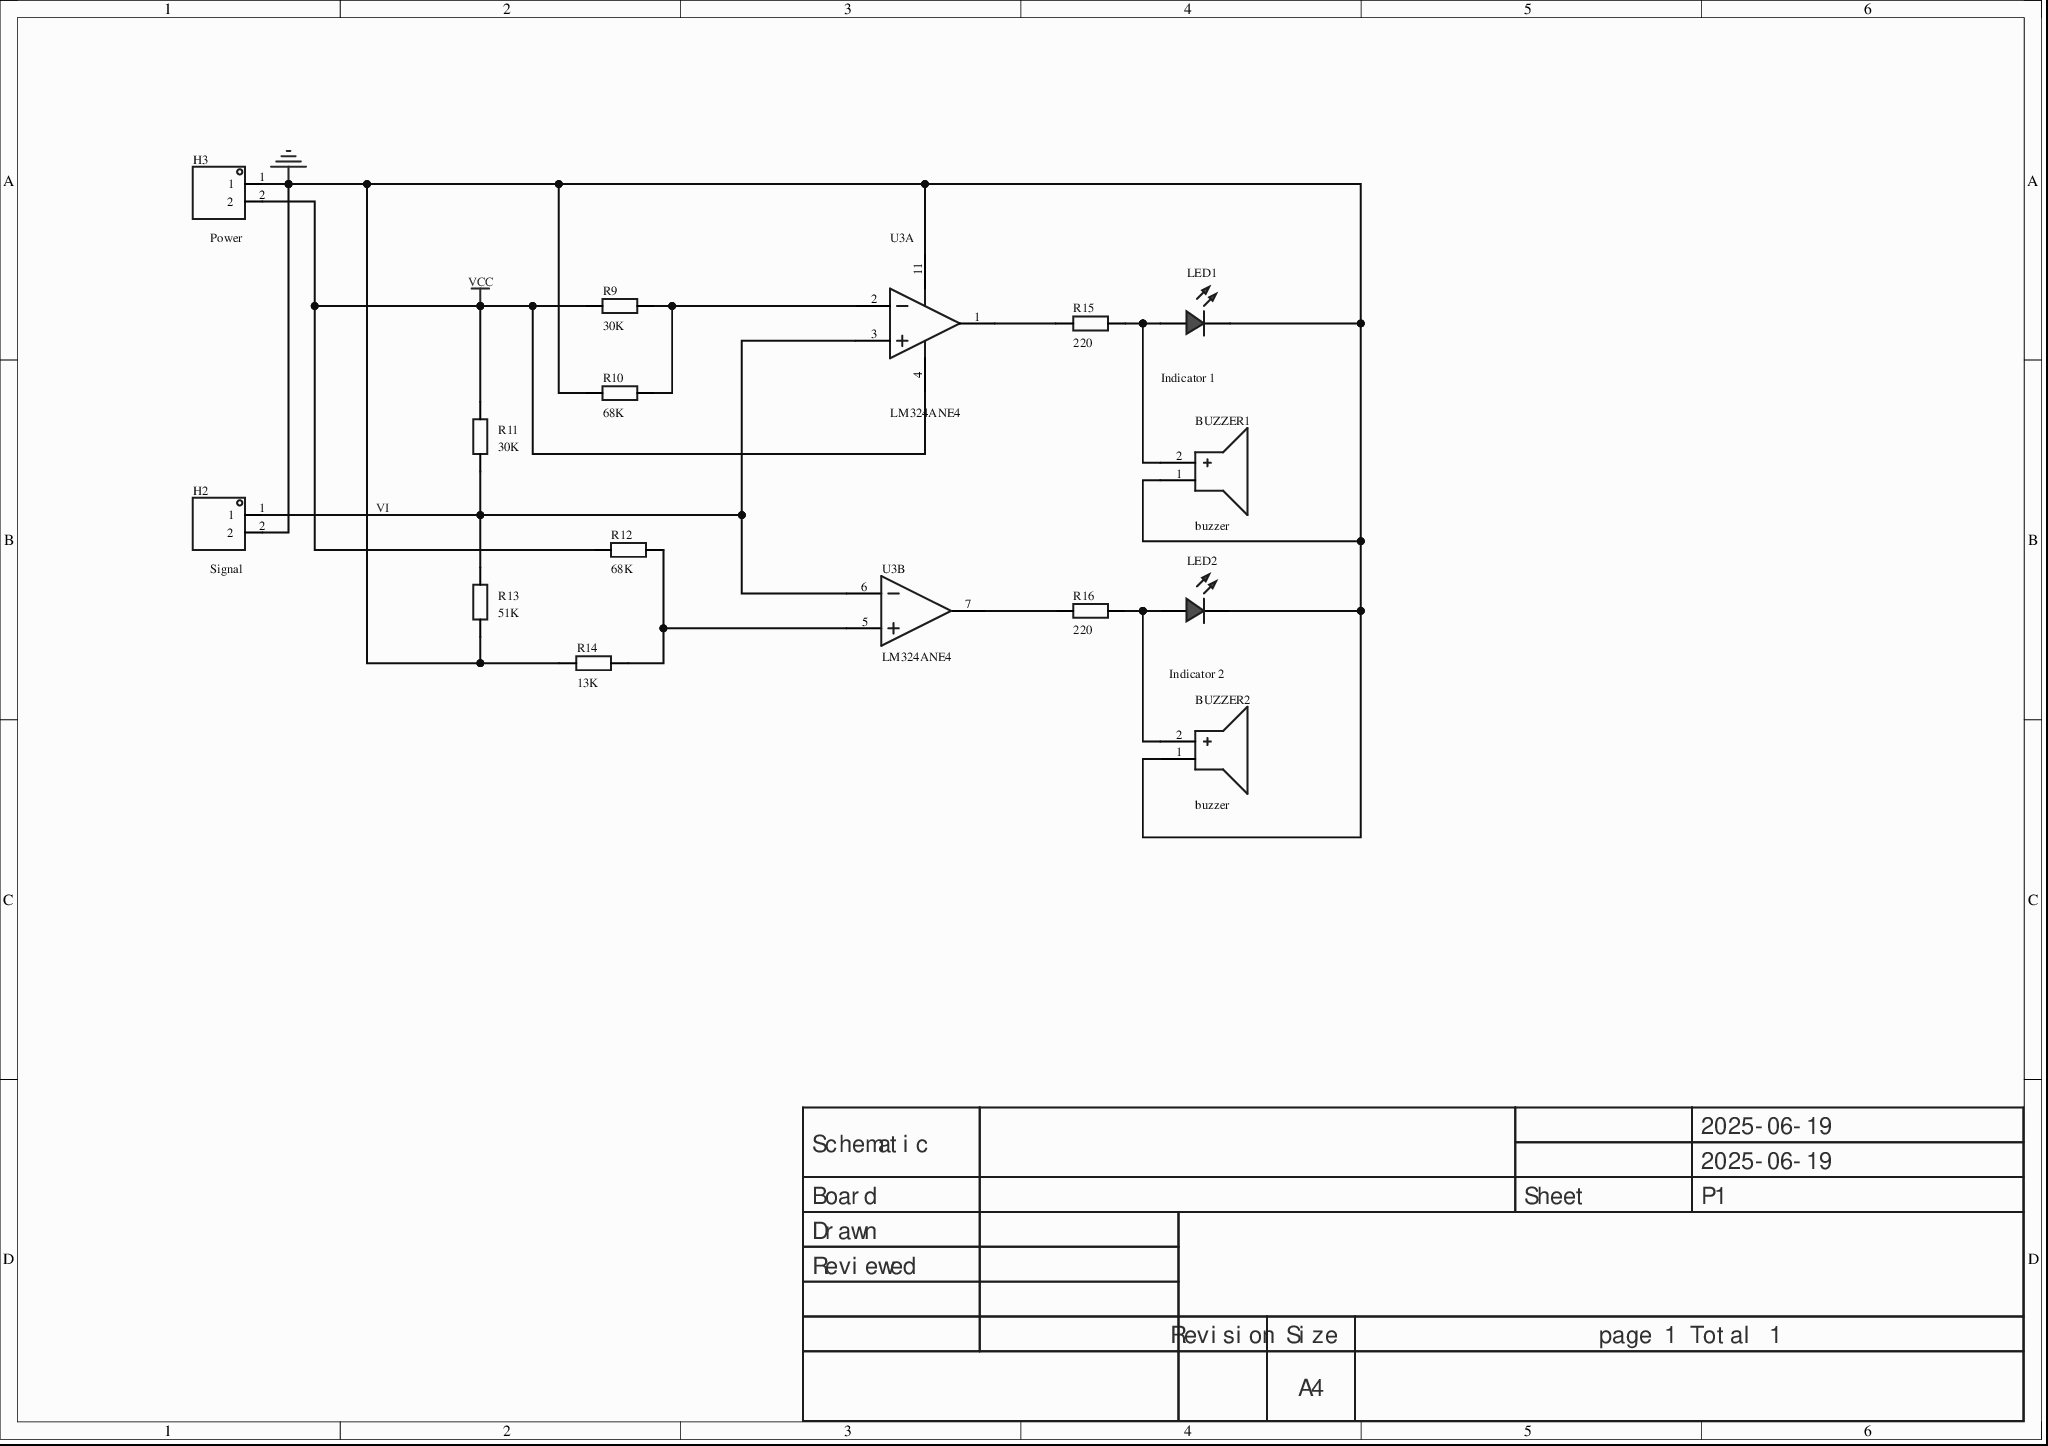
[diagram p0: MISC51341-3.schdoc]
# Altium project MISC51341-2.PrjPcb
1 sheet, 15 parts. Net scope: global (net labels, ports and power ports of the same name join across sheets).
Board file: MISC51341.pcbdoc

## Sheet MISC51341-3.schdoc
size 297 x 209 mm; Version: V1.0; @Project Name: MISC51341; @Page Count: 1; @Update Date: 2025-06-19; @Create Date: 2025-06-19; @Schematic Name: MISC51341; @Page No: 1; @Create Time: 16:02:31; @Update Time: 16:31:31; @Board Name: MISC51341

### Parts
BUZZER1  buzzer  [BUZ-TH_BD12.0-P6.00-D0.9-RD]
BUZZER2  buzzer  [BUZ-TH_BD12.0-P6.00-D0.9-RD]
H2  (no value)  [HDR-TH_2P-P2.54-V-M-1]
H3  (no value)  [HDR-TH_2P-P2.54-V-M-1]
LED1  (no value)  [LED_TH-3mm]
LED2  (no value)  [LED_TH-3mm]
R9  30K  [Res_1/8W]
R10  68K  [Res_1/8W]
R11  30K  [Res_1/8W]
R12  68K  [Res_1/8W]
R13  51K  [Res_1/8W]
R14  13K  [Res_1/8W]
R15  220  [Res_1/8W]
R16  220  [Res_1/8W]
U3  LM324ANE4  [PDIP-14_L19.6-W6.5-P2.54-LS7.9-BL]  (parts A,B of 4)

### Nets
GND: BUZZER1.1(-) BUZZER2.1(-) H2.2 H3.1 LED1.2(A) LED2.2(A) R10.1 R13.1 R14.1 U3.11(GND)
VCC: H3.2 R9.1 R11.2 R12.1 U3.4(VCC)
VI: H2.1 R11.1 R13.2 U3.3(IN1-) U3.6(IN2-)
NetBUZZER1_2: BUZZER1.2(+) LED1.1(C) R15.2
NetBUZZER2_2: BUZZER2.2(+) LED2.1(C) R16.2
NetR9_2: R9.2 R10.2 U3.2(IN1+)
NetR12_2: R12.2 R14.2 U3.5(IN2+)
NetR15_1: R15.1 U3.1(OUT1)
NetR16_1: R16.1 U3.7(OUT2)

### Notes on the sheet
- (near H3) Power
- Indicator 1
- (near H2) Signal
- Indicator 2
- 2025-06-19
- Schematic
- Board
- Sheet
- P1
- Drawn
- Reviewed
- Revision
- Size
- A4
- page 1 Total 1

### Library data of the parts
BUZZER1 BUZZER2 = buzzer: AddInBom: yes; ModelId: af17e4151ed84fc2a628230bf2376363; ModelTransform: 472.44,472.176,0,270,0,0,0,0,-196.85; Symbol: BUZZER; Device: buzzer; LCSC Part Name: buzzer; SupplierPart: C9900014030; ManufacturerPart: buzzer; Supplier Footprint: buzzer; JLCPCB Part Class: Extended Part; Supplier: LCSC; ConvertToPcb: yes; FootprintName: BUZ-TH_BD12.0-P6.00-D0.9-RD; ModelName: BUZ-TH_BD12.0-P6.00-D0.9-RD
H2 H3 = HDR-M_2.54_1x2P: Symbol: 210S-1*2P L=11.6MMGold-plated black; ConvertToPcb: yes; ModelId: 79b2e9f2d70a4d68a1b7098f27c6d4c5; ModelName: HDR-M-2.54_1x2; ModelTransform: 200,100,0,0,0,0,0,0,-118.11; Device: HDR-M_2.54_1x2P; AddInBom: yes; SupplierPart: C124375; Supplier Footprint: 插件; FootprintName: HDR-TH_2P-P2.54-V-M-1
LED1 LED2 = LED_TH-R_3mm: ConvertToPcb: yes; ModelId: a497c992633541038a38947cdc58012f; ModelName: LED-TH-3mm_R; ModelTransform: 141.274,153.327,0,0,0,0,-5.984,0,-137.795; Symbol: LED_TH-R; Device: LED_TH-R_3mm; AddInBom: yes; FootprintName: LED_TH-3mm; Supplier Footprint: 插件
R9-R16 = Res_AXIAL-1/8W: ConvertToPcb: yes; SymbolName: Resistor; ModelId: b2b5ae7ae4c642178fe0039925c86a3f; ModelName: RES-TH_BD1.8-L3.2-P7.20-D0.4; ModelTransform: 282.86,66.88,253.09,0,0,0,0,0,-191; Device: Res_AXIAL-1/8W; AddInBom: yes; Supplier Footprint: 轴向引线; FootprintName: Res_1/8W
  R9 R11: Value: 30K
  R10 R12: Value: 68K
  R13: Value: 51K
  R14: Value: 13K
  R15 R16: Value: 220
U3 = LM324ANE4: Manufacturer: TI(德州仪器); Relevance: []; AddInBom: yes; ModelId: 9c02f2b186e4457baa67e0f5e04a653b; ModelName: PDIP-14_L19.6-W6.5-H5.1-P2.54-LS7.9-BL; ModelTransform: 771.652,311.8104,0,0,0,0,0,0,-118.11; Symbol: LM324ANE4; Device: LM324ANE4; LCSC Part Name: LM324ANE4; SupplierPart: C4369463; ManufacturerPart: LM324ANE4; Supplier Footprint: PDIP-14; JLCPCB Part Class: Extended Part; Datasheet: https://atta.szlcsc.com/upload/public/pdf/source/20230921/F20B5F7192F3313CCC48B830029C6C49.pdf; Supplier: LCSC; ConvertToPcb: yes; FootprintName: PDIP-14_L19.6-W6.5-P2.54-LS7.9-BL